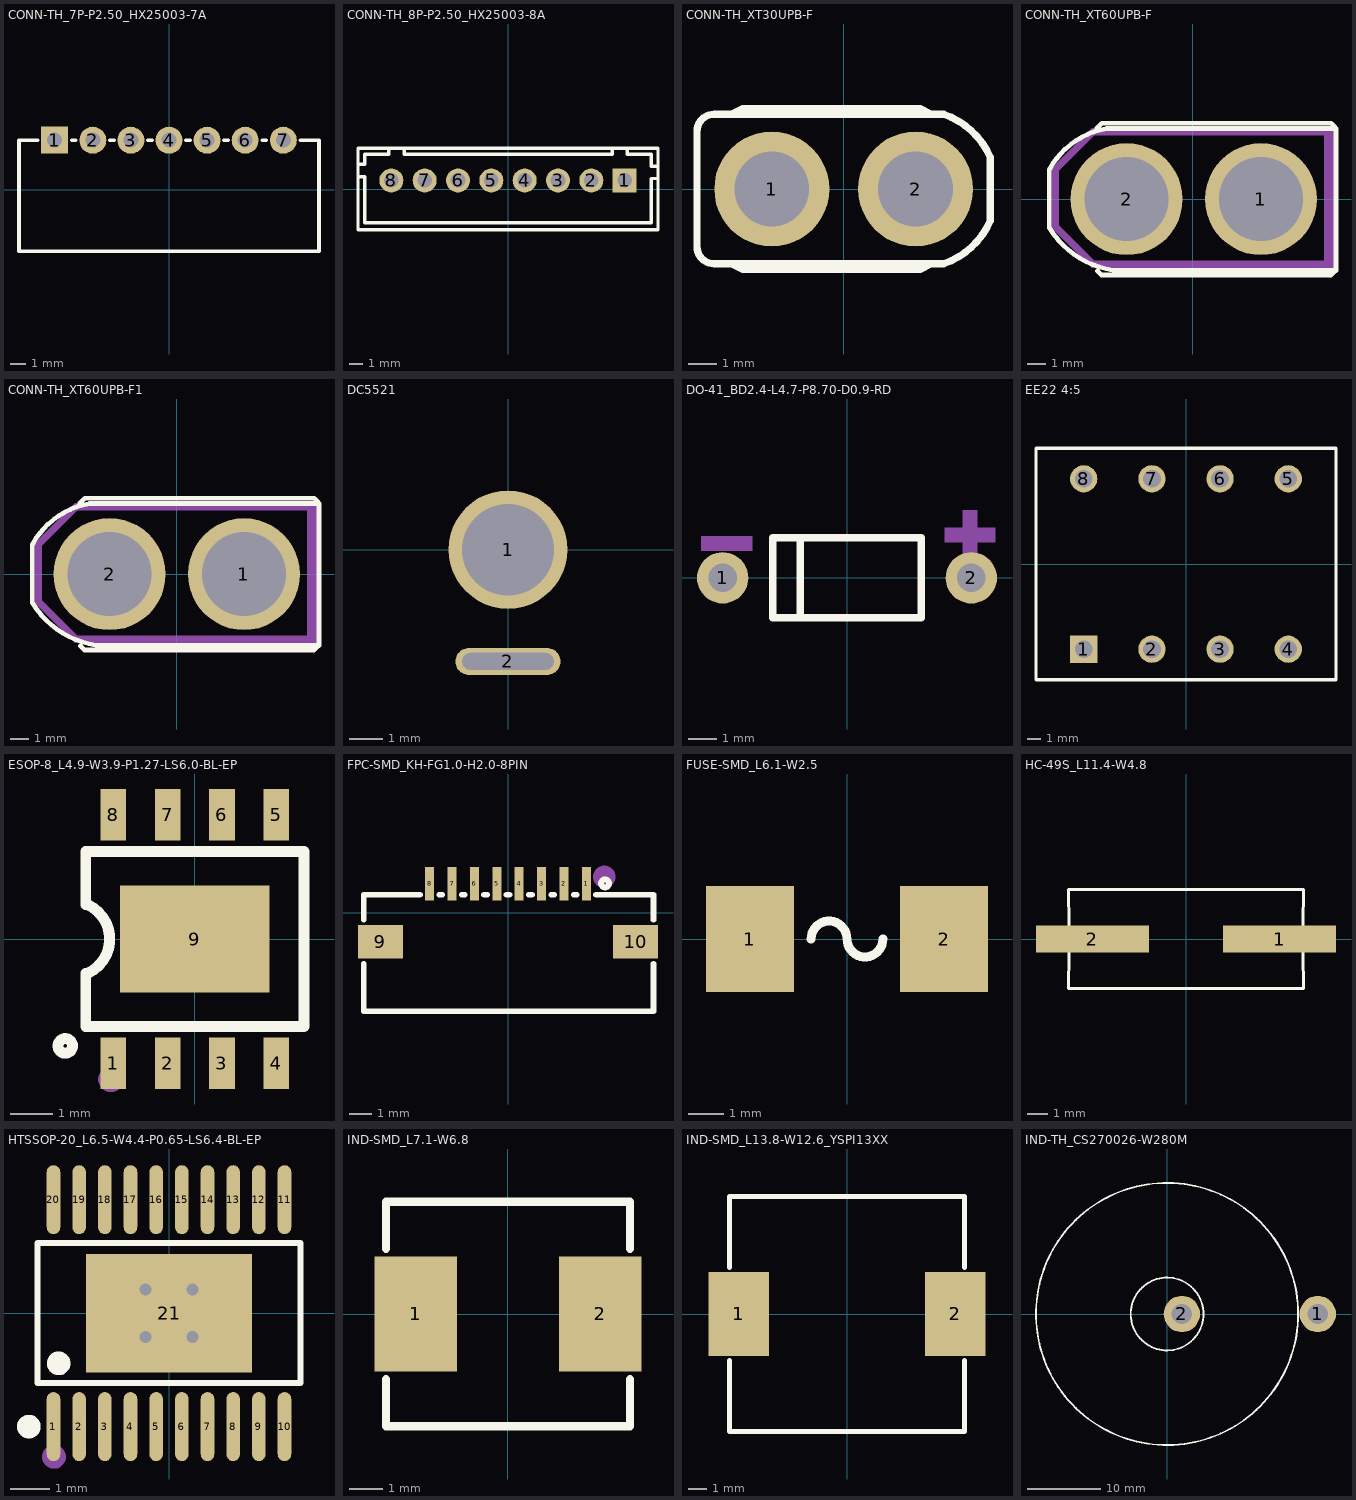
[diagram p0: the footprints below, top view; thin cyan lines are the x and y axes]
# Altium footprint library MISC84402-2.PcbLib: 69 footprints (part 2 of 5)
Each footprint in its own frame and in the unit in brackets; x right, y up, seen from the top. Pads: shape width x height; smd on the part's side, far side on the other; paste and mask are expansions set on the pad; w line width, h text height; cw(c..) or ccw(c..) is an arc to the next point about the centre after c.

## CONN-TH_7P-P2.50_HX25003-7A [mm]
pads (7):
  rect 1.8x1.8 hole 1: 1(-7.62,3.314)
  round 1.8 hole 1: 2(-5.08,3.314) 3(-2.54,3.314) 4(0,3.314) 5(2.54,3.314) 6(5.08,3.314) 7(7.62,3.314)
Top Overlay:
  lines w0.254: -8.751,3.314 -10,3.314 -10,-4.087 10,-4.087 10,3.314 8.751,3.314 ; -6.489,3.314 -6.211,3.314 ; -3.949,3.314 -3.671,3.314 ; -1.409,3.314 -1.131,3.314 ; 1.131,3.314 1.409,3.314 ; 3.671,3.314 3.949,3.314 ; 6.211,3.314 6.489,3.314

## CONN-TH_8P-P2.50_HX25003-8A [mm]
pads (8):
  rect 1.8x1.8 hole 1.1: 1(8.75,0.646)
  round 1.8 hole 1.1: 2(6.25,0.646) 3(3.75,0.646) 4(1.25,0.646) 5(-1.25,0.646) 6(-3.75,0.646) 7(-6.25,0.646) 8(-8.75,0.646)
Top Overlay:
  lines w0.254: -11.25,0.915 -10.75,0.915 -10.75,-2.521 10.749,-2.521 10.749,0.786 11.249,0.786 ; -11.25,1.845 -10.75,1.845 -10.75,2.604 -8.944,2.604 -8.944,3.054 ; -7.8,2.604 7.8,2.604 ; -7.793,2.601 -7.793,3.05 ; 7.807,2.601 7.807,3.05 ; 8.943,2.604 10.749,2.604 10.749,1.715 11.249,1.715 ; 8.95,2.602 8.95,3.05 ; -11.25,-3.054 -11.25,3.046 11.25,3.046 11.25,-3.054 -11.25,-3.054

## CONN-TH_XT30UPB-F [mm]
pads (2):
  round 4 hole 2.6: 1(-2.5,0) 2(2.5,0)
Top Overlay:
  lines w0.254: -3.9,-2.6 -3.5,-2.8 2.65,-2.8 3.05,-2.6 ; -3.9,2.6 -3.5,2.8 2.65,2.8 3.05,2.6 ; -5.1,-2 ccw(c-4.5,-2) -4.5,-2.6 3.475,-2.6 ccw(c2.58,0) 5.1,-1.1 5.1,1.1 ccw(c2.58,0) 3.475,2.6 -4.5,2.6 ccw(c-4.5,2) -5.1,2 -5.1,-2

## CONN-TH_XT60UPB-F [mm]
pads (2):
  round 6 hole 4.5: 1(3.663,0) 2(-3.536,0)
Top Overlay:
  lines w0.254: -7.683,-1.524 -7.683,1.576 cw(c-3.873,-0.482) -4.625,3.783 7.683,3.783 7.683,-3.819 ; -7.668,-1.548 ccw(c-3.507,1.016) -4.283,-3.81 7.658,-3.81 ; -5.119,3.819 -4.874,4.064 -4.827,4.064 7.419,4.064 7.638,3.844 ; -5.099,-3.844 -4.88,-4.064 7.365,-4.064 7.413,-4.064 7.658,-3.819
Mechanical 15:
  region: 7.556,3.429 7.556,-3.302 7.048,-3.302 7.048,3.429
  region: -5.397,-3.683 -5.397,-3.302 7.556,-3.302 7.556,-3.683
  region: -5.397,3.81 7.556,3.81 7.556,3.429 -5.271,3.429
  region: -7.556,1.651 -7.556,-1.524 -7.175,-1.524 -7.175,1.651
  region: -7.556,-1.524 -5.397,-3.683 -5.143,-3.429 -7.302,-1.27
  region: -5.397,3.81 -7.556,1.651 -7.302,1.397 -5.143,3.556

## CONN-TH_XT60UPB-F1 [mm]
pads (2):
  round 6 hole 4.5: 1(3.6,0) 2(-3.6,0)
Top Overlay:
  lines w0.254: -7.747,-1.524 -7.747,1.576 cw(c-3.937,-0.482) -4.689,3.782 7.62,3.782 7.62,-3.819 ; -7.732,-1.548 ccw(c-3.57,1.016) -4.346,-3.81 7.595,-3.81 ; -5.183,3.819 -4.938,4.064 -4.89,4.064 7.355,4.064 7.575,3.844 ; -5.163,-3.844 -4.943,-4.064 7.302,-4.064 7.35,-4.064 7.595,-3.819
Mechanical 15:
  region: -5.461,3.81 -7.62,1.651 -7.366,1.397 -5.207,3.556
  region: -7.62,-1.524 -5.461,-3.683 -5.207,-3.429 -7.366,-1.27
  region: -7.62,1.651 -7.62,-1.524 -7.239,-1.524 -7.239,1.651
  region: -5.461,3.81 7.493,3.81 7.493,3.429 -5.334,3.429
  region: -5.461,-3.683 -5.461,-3.302 7.493,-3.302 7.493,-3.683
  region: 7.493,3.429 7.493,-3.302 6.985,-3.302 6.985,3.429

## DC5521 [mm]
pads (2):
  round 3.5 hole 2.7: 1(0,0)
  oval 3.1x0.8 hole 0.5 slot 2.7 at 0 deg: 2(0,-3.302)
Bottom Overlay:
  circle w0.254: c0,0 r4

## DO-41_BD2.4-L4.7-P8.70-D0.9-RD [mm]
pads (2):
  round 1.8 hole 1: 1(-4.35,0) 2(4.35,0)
Top Overlay:
  lines w0.254: -1.641,-1.4 -1.641,1.4 ; -2.6,-1.4 2.6,-1.4 2.6,1.4 -2.6,1.4 -2.6,-1.4
Mechanical 15:
  region: 3.415,1.759 5.193,1.759 5.193,1.251 3.415,1.251
  region: 4.045,0.593 4.045,2.371 4.553,2.371 4.553,0.593
  region: -5.102,1.451 -3.324,1.451 -3.324,0.943 -5.102,0.943

## EE22 4:5 [mm]
pads (8):
  rect 2x2 hole 1.3: 1(-7.5,-6.25)
  round 2 hole 1.3: 2(-2.5,-6.25) 3(2.5,-6.25) 4(7.5,-6.25) 5(7.5,6.25) 6(2.5,6.25) 7(-2.5,6.25) 8(-7.5,6.25)
Top Overlay:
  lines w0.254: -11,-8.5 -11,8.5 11,8.5 11,-8.5 -11,-8.5

## ESOP-8_L4.9-W3.9-P1.27-LS6.0-BL-EP [mm]
pads (9):
  rect 0.6x1.2 smd: 1(-1.905,-2.908) 2(-0.635,-2.908) 3(0.635,-2.908) 4(1.905,-2.908) 5(1.905,2.908) 6(0.635,2.908) 7(-0.635,2.908) 8(-1.905,2.908)
  rect 3.5x2.5 smd: 9(0,0)
Top Overlay:
  circle w0.254: c-3.03,-2.5 r0.17
  lines w0.254: -2.55,-0.8 -2.55,-2.05 2.55,-2.05 2.55,2.05 -2.55,2.05 -2.55,0.8 ; -2.5,-0.8 ccw(c-2.875,0) -2.5,0.8
Mechanical 15:
  circle w0.3: c-1.96,-3.28 r0.15

## FPC-SMD_KH-FG1.0-H2.0-8PIN [mm]
pads (10):
  rect 0.4x1.5 smd: 1(3.5,1.3) 2(2.5,1.3) 3(1.5,1.3) 4(0.5,1.3) 5(-0.5,1.3) 6(-1.5,1.3) 7(-2.5,1.3) 8(-3.5,1.3)
  rect 2x1.5 smd: 9(-5.7,-1.3) 10(5.7,-1.3)
Top Overlay:
  circle w0.254: c4.335,1.308 r0.18
  lines w0.254: -6.45,-2.281 -6.45,-4.4 6.5,-4.4 6.5,-2.281 ; -6.45,-0.319 -6.45,0.8 -3.931,0.8 ; -3.069,0.8 -2.931,0.8 ; -2.069,0.8 -1.931,0.8 ; -1.069,0.8 -0.931,0.8 ; -0.069,0.8 0.069,0.8 ; 0.931,0.8 1.069,0.8 ; 1.931,0.8 2.069,0.8 ; 2.931,0.8 3.069,0.8 ; 3.931,0.8 6.5,0.8 6.5,-0.319
Mechanical 15:
  circle w0.5: c4.3,1.6 r0.25

## FUSE-SMD_L6.1-W2.5 [mm]
pads (2):
  rect 2.5x3 smd: 1(-2.75,0) 2(2.75,0)
Top Overlay:
  lines w0.254: -1.016,0 cw(c-0.508,0) 0,0 ccw(c0.508,0) 1.016,0

## HC-49S_L11.4-W4.8 [mm]
pads (2):
  rect 5.5x1.3 smd: 1(4.553,0) 2(-4.553,0)
Top Overlay:
  lines w0.152: -5.715,-2.413 -5.7,-0.662 -5.715,-2.413 ; -5.715,-2.413 5.715,-2.413 ; -5.715,-2.413 5.715,-2.413 ; -5.715,2.413 5.715,2.413 ; -5.715,2.413 -5.7,0.662 -5.715,2.413 ; -5.715,2.413 5.715,2.413 ; 5.715,-2.413 5.7,-0.662 5.715,-2.413 ; 5.715,2.413 5.7,0.662 5.715,2.413

## HTSSOP-20_L6.5-W4.4-P0.65-LS6.4-BL-EP [mm]
pads (21):
  oval 0.343x1.747 smd: 1(-2.925,-2.873) 2(-2.275,-2.873) 3(-1.625,-2.873) 4(-0.975,-2.873) 5(-0.325,-2.873) 6(0.325,-2.873) 7(0.975,-2.873) 8(1.625,-2.873) 9(2.275,-2.873) 10(2.925,-2.873) 11(2.925,2.873) 12(2.275,2.873) 13(1.625,2.873) 14(0.975,2.873) 15(0.325,2.873) 16(-0.325,2.873) 17(-0.975,2.873) 18(-1.625,2.873) 19(-2.275,2.873) 20(-2.925,2.873)
  rect 4.2x3 smd: 21(0,0)
via 0.6,0.6 diameter 0.61 hole 0.305
via -0.6,0.6 diameter 0.61 hole 0.305
via -0.6,-0.6 diameter 0.61 hole 0.305
via 0.6,-0.6 diameter 0.61 hole 0.305
Top Overlay:
  circle w0.3: c-3.549,-2.873 r0.15
  circle w0.3: c-2.794,-1.27 r0.15
  lines w0.152: -3.326,-1.771 -3.326,1.771 3.326,1.771 3.326,-1.771 -3.326,-1.771
Mechanical 15:
  circle w0.3: c-2.912,-3.638 r0.15

## IND-SMD_L7.1-W6.8 [mm]
pads (2):
  rect 2.5x3.5 smd: 1(-2.8,0) 2(2.8,0)
Top Overlay:
  lines w0.254: -3.7,-1.981 -3.7,-3.4 3.7,-3.4 3.7,-1.981 ; -3.7,1.981 -3.7,3.4 3.7,3.4 3.7,1.981

## IND-SMD_L13.8-W12.6_YSPI13XX [mm]
pads (2):
  rect 3.25x4.5 smd: 1(-5.8,0) 2(5.8,0)
Top Overlay:
  lines w0.254: -6.3,-2.481 -6.3,-6.3 6.3,-6.3 6.3,-2.481 ; -6.3,2.481 -6.3,6.3 6.3,6.3 6.3,2.481

## IND-TH_CS270026-W280M [mm]
pads (2):
  round 5 hole 2.8: 1(20.701,0) 2(2.032,0)
Top Overlay:
  circle w0.254: c0,0 r18
  circle w0.254: c0,0 r5